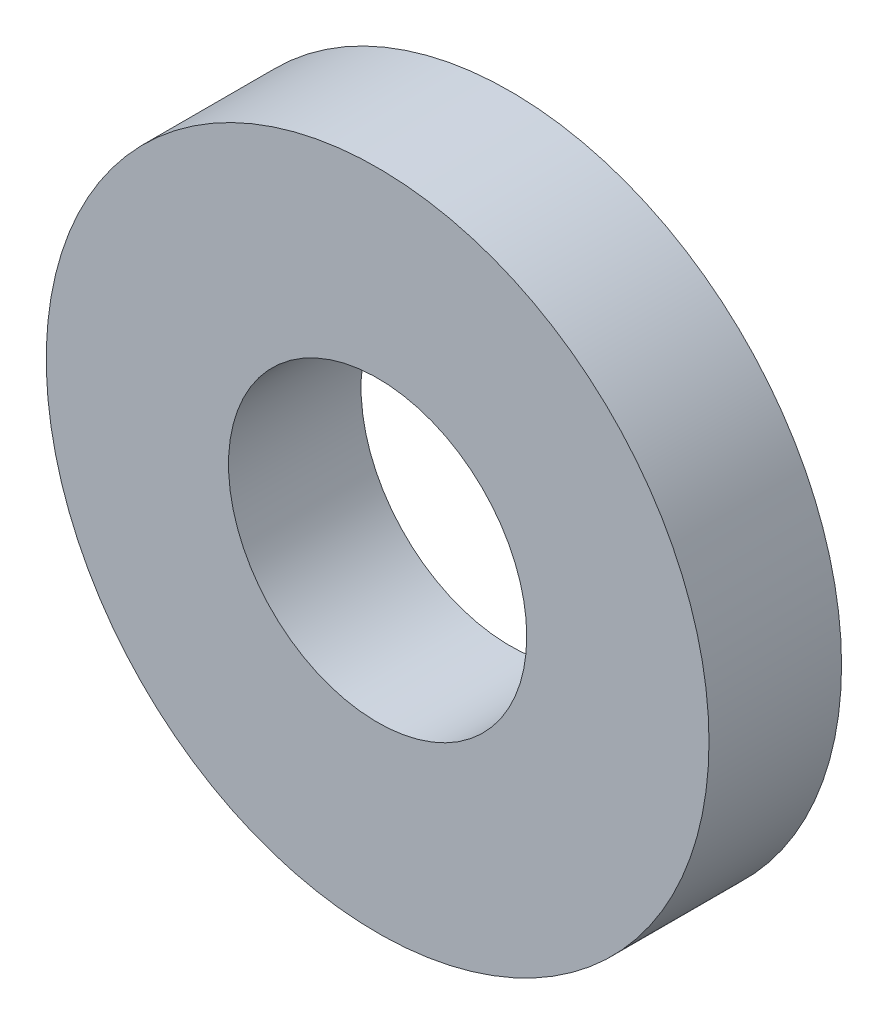
from build123d import *

# Parameters (mm, degrees)
SKETCH_1_R      = 10
SKETCH_1_R_2    = 4.5
EXTRUDE_1_DEPTH = 4


with BuildPart() as part:
    # 草图1 → 凸台-拉伸1 (new body)
    with BuildSketch(Plane.XY):
        Circle(SKETCH_1_R)
        Circle(SKETCH_1_R_2, mode=Mode.SUBTRACT)
    extrude(amount=EXTRUDE_1_DEPTH)


solid = part.part
